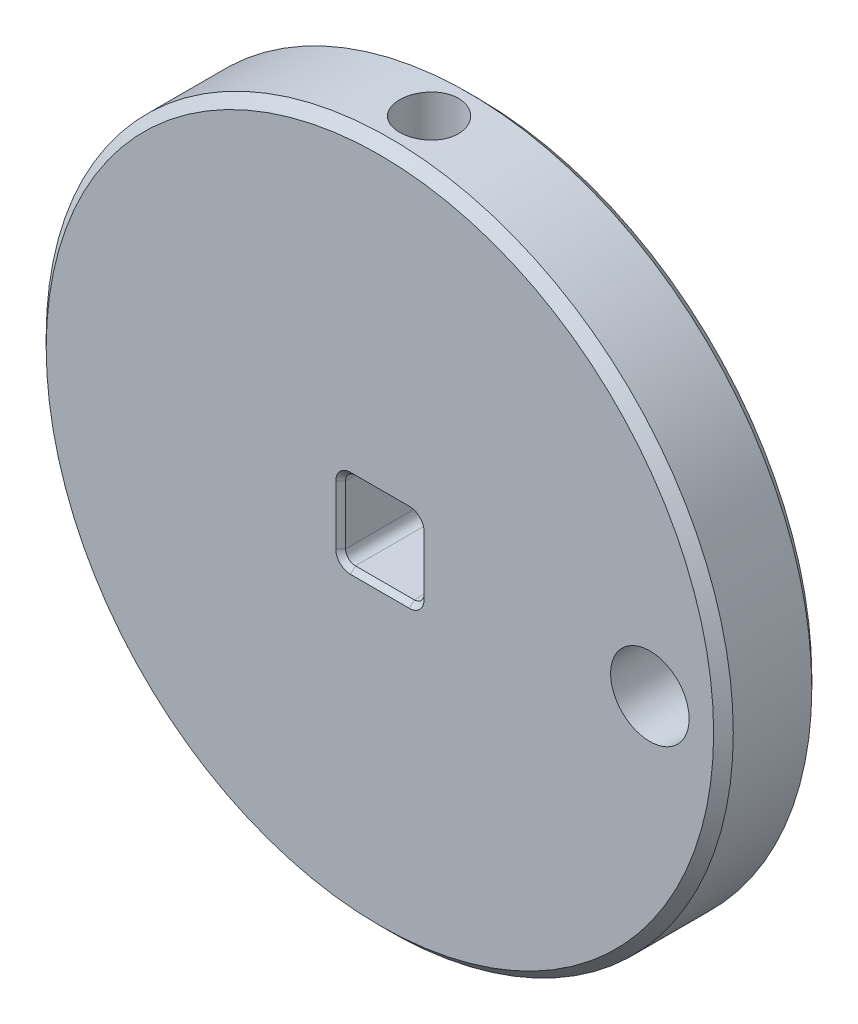
SolidWorks part; units mm, degrees
ref_plane "Front Plane" through (0, 0, 0) normal (0, 0, 1) x (1, 0, 0)
ref_plane "Top Plane" through (0, 0, 0) normal (0, 1, 0) x (1, 0, 0)
ref_plane "Right Plane" through (0, 0, 0) normal (1, 0, 0) x (0, 0, -1)
sketch "Sketch1" plane through (0, 0, 0) normal (0, 0, 1) x (1, 0, 0)
  circle A0 centre (0, 0) radius 35
  dimension "D1" = 70
extrude "Boss-Extrude1" add sketch "Sketch1" along normal blind 10
chamfer "Chamfer1" distance 1 angle 45 2 edges at (35, 0, 0) (35, 0, 10)
sketch "Sketch2" plane through (0, 0, 10) normal (0, 0, 1) x (1, 0, 0)
  circle A0 centre (0, 0) radius 1
  dimension "D1" = 2
extrude "Cut-Extrude1" cut sketch "Sketch2" against normal blind 30
sketch "Sketch3" plane through (0, 0, 10) normal (0, 0, 1) x (1, 0, 0)
  circle A1 centre (27.5, 0) radius 4
  dimension "D2" = 8
extrude "Cut-Extrude2" cut sketch "Sketch3" against normal blind 29
sketch "Sketch4" plane through (0, 0, 10) normal (0, 0, 1) x (1, 0, 0)
  line L1 (-4, 4) -> (4, 4)
  line L2 (-4, 4) -> (-4, -4)
  line L3 (-4, -4) -> (4, -4)
  line L4 (4, 4) -> (4, -4)
  line L5 (-4, 4) -> (4, -4) construction
  line L6 (-4, -4) -> (4, 4) construction
  point P0 (0, 0)
  dimension "D1" = 8
  dimension "D2" = 8
extrude "Cut-Extrude3" cut sketch "Sketch4" against normal through all
fillet "Fillet1" radius 1 4 edges at (-4, -4, 5) (4, -4, 5) (4, 4, 5) (-4, 4, 5)
sketch "Sketch5" plane through (0, 4, 0) normal (0, -1, 0) x (1, 0, 0)
  line L0 (0, 0) -> (0, 10) construction
  line L1 (34, 10) -> (-34, 10) construction
  circle A0 centre (0, 5) radius 0.5
  dimension "D1" = 1
extrude "Cut-Extrude4" cut sketch "Sketch5" against normal through all
ref_plane "Plane1" through (0, 14, 0) normal (0, 1, 0) x (1, 0, 0)
sketch "Sketch7" plane through (0, 14, 0) normal (0, 1, 0) x (1, 0, 0)
  circle A0 centre (0, -5) radius 3
  dimension "D1" = 6
extrude "Cut-Extrude5" cut sketch "Sketch7" along normal through all
hole_wizard "M3 Tapped Hole1" positions "3DSketch2" profile "Sketch8" tap size "M3" standard "GB"
sketch3d "3DSketch2"
  line L0 (0, 14, 5) -> (0, 4, 5) construction
  point P0 (0, 14, 5)
sketch "Sketch8" plane through (0, 14, 5) normal (1, 0, 0) x (0, 0, 1)
  line L0 (0, 0) -> (0, 12.7511)
  line L1 (0, 12.7511) -> (1.25, 12)
  line L2 (1.25, 12) -> (1.25, 0)
  line L5 (1.25, 0) -> (0, 0)
  line L10 (0, 12.7511) -> (-1.25, 12) construction
  line L11 (0, -6.35) -> (0, 107.95) construction
  dimension "螺纹孔钻头直径" = 2.5
  dimension "螺纹孔钻头深度" = 12
  dimension "导头角度" = 118
cosmetic thread "Cosmetic thread 1" parameters "D1"=10, "D2"=3
chamfer "Chamfer2" distance 0.5 angle 45 16 edges at (0, -4, 0) (3.7071, -3.7071, 0) (-3.7071, -3.7071, 0) (4, 0, 0) (-4, 0, 0) (3.7071, 3.7071, 0) (-3.7071, 3.7071, 0) (0, 4, 0) (4, 0, 10) (3.7071, 3.7071, 10) (3.7071, -3.7071, 10) (0, 4, 10) (0, -4, 10) (-3.7071, 3.7071, 10) (-3.7071, -3.7071, 10) (-4, 0, 10)
